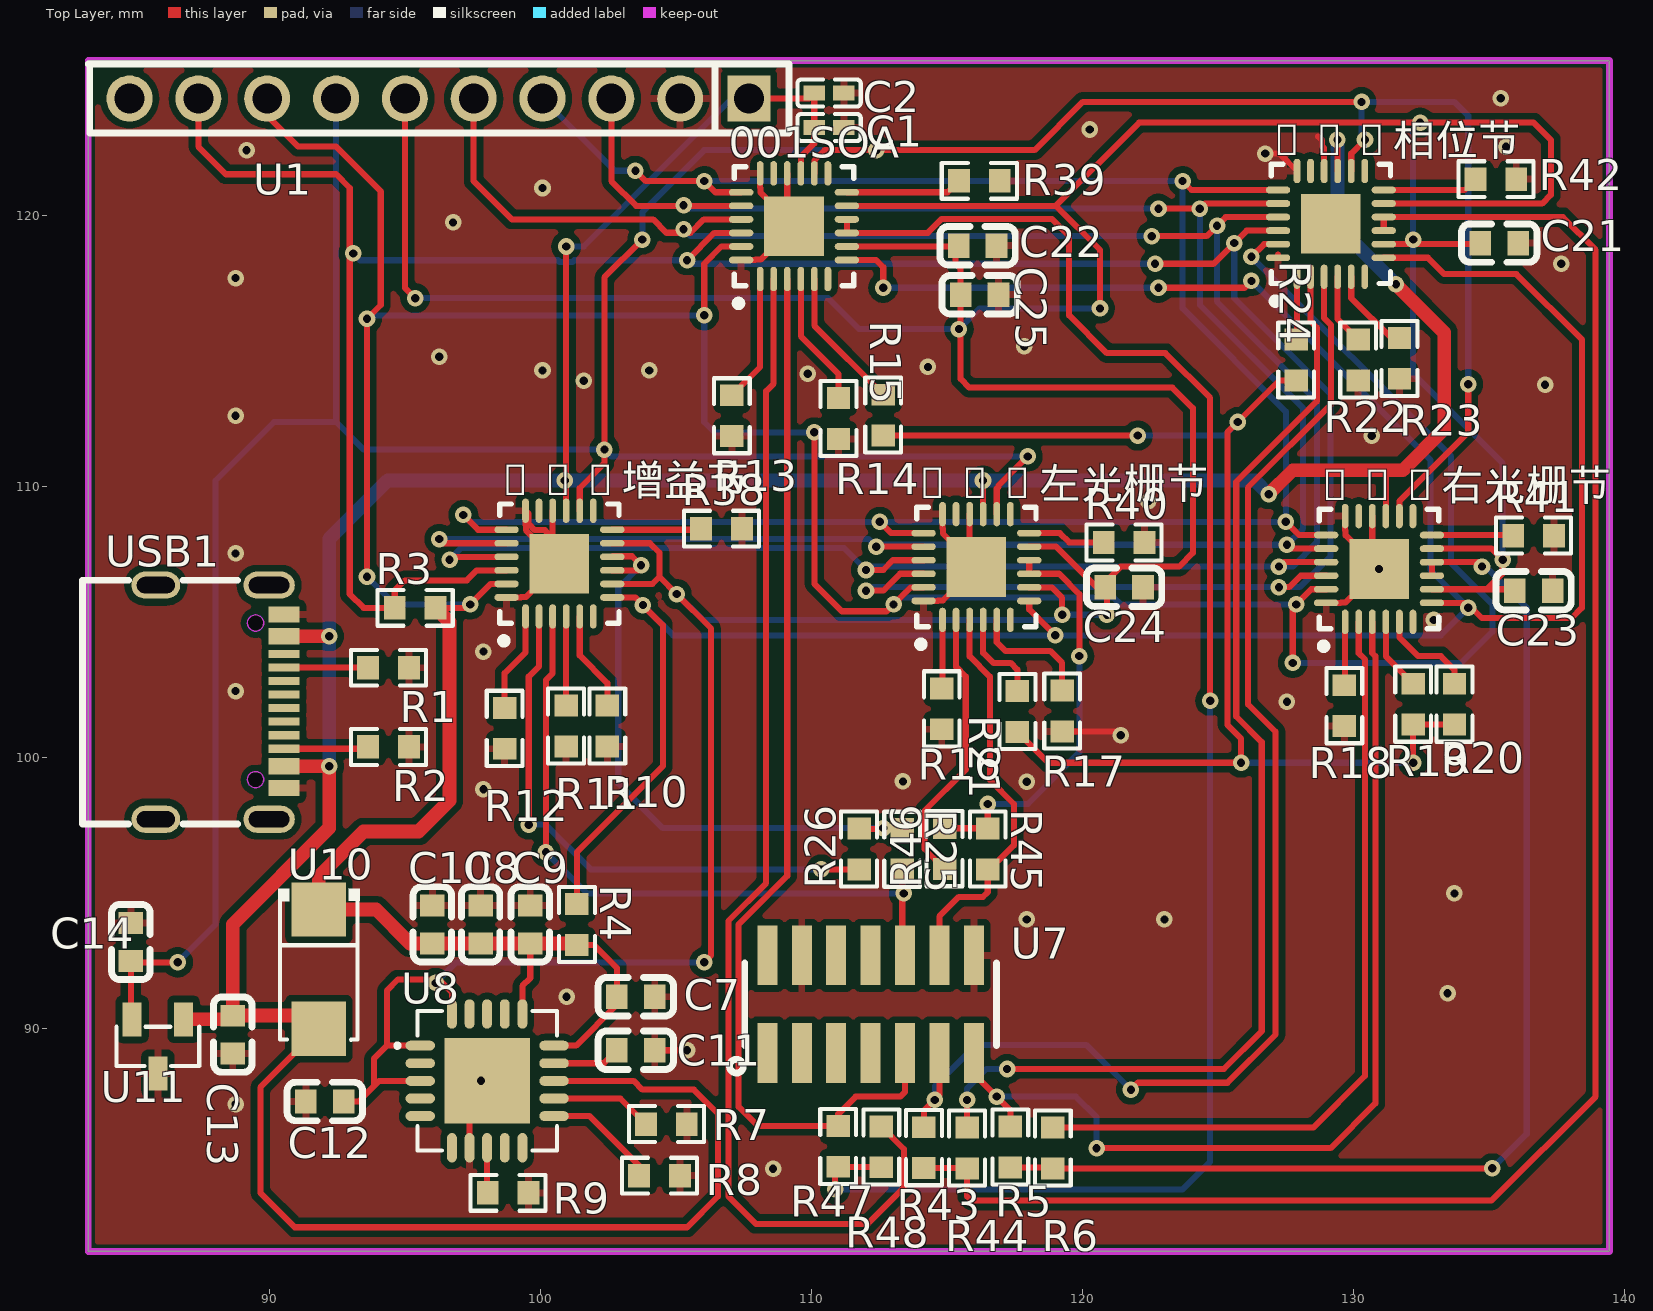
[diagram p0: Top Layer view]
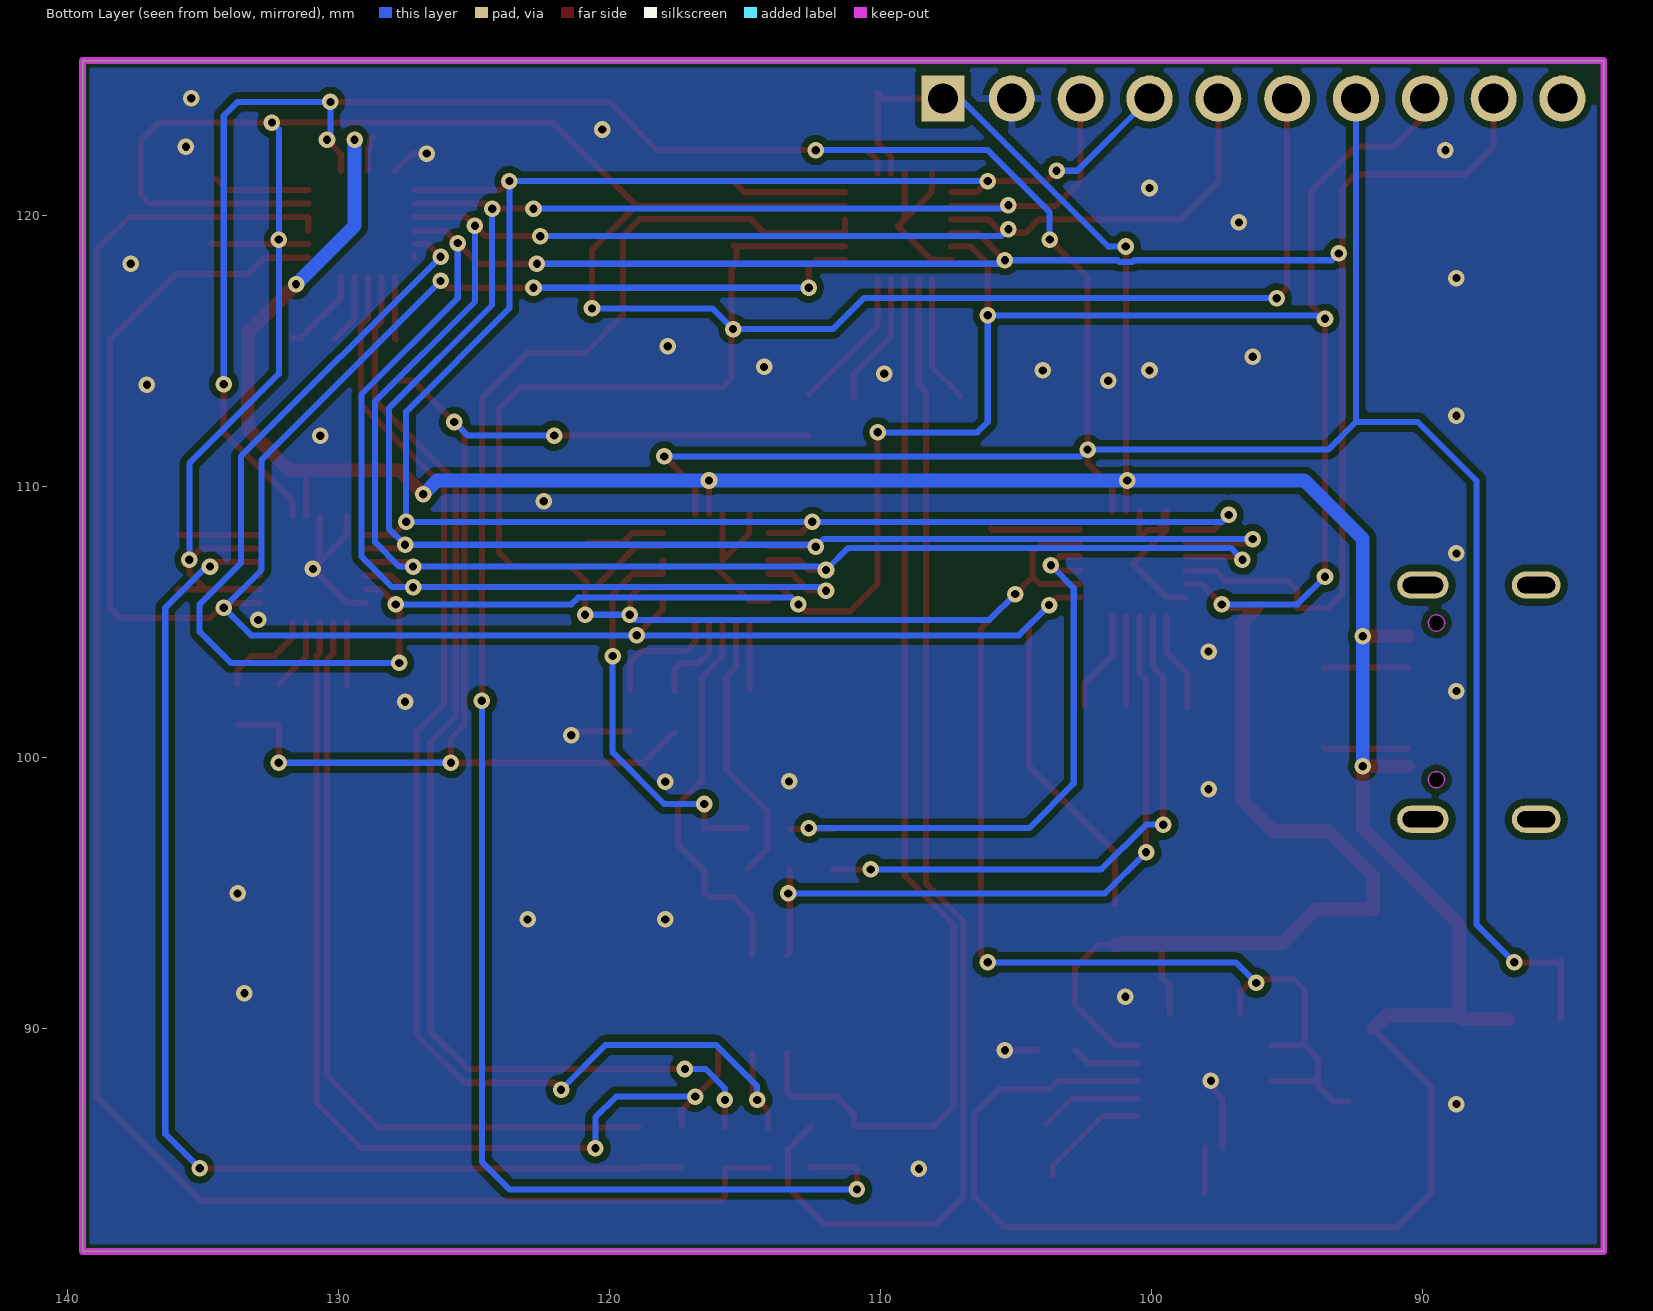
[diagram p1: Bottom Layer view, seen from below]
# Altium PCB MISC49910.pcbdoc
Units mm, origin at the board's own origin, x right, y up, seen from the top; angles counter-clockwise.
Board outline 56.13 x 43.94 mm, 2 copper layers (Top Layer, Bottom Layer), stack 1.58 mm thick; 63 components, 53 nets, 295 pads, 127 vias.

## Layer stack, top to bottom
Top Solder Mask Layer: solder mask 0.01, Dk 3.3
Top Layer: signal copper 0.035
Dielectric1: surface 1.51, FR4, Dk 4.5
Bottom Layer: signal copper 0.035
Bottom Solder Mask Layer: solder mask 0.01, Dk 3.3

## Board outline
83.312,125.73 83.312,81.788 139.446,81.788 139.446,125.73

## Design rules (kind name [scope] priority, off if disabled: settings)
BoardOutlineClearance copperThickness2oz_1 [All] p2 off: genericclearance=0.203 ignorepadtopadclearanceinfootprint=FALSE except(0: Arc-SplitContinuation Track-SplitContinuation SMDPad-SplitContinuation THPad-SplitContinuation Via-SplitContinuation Fill-SplitContinuation Region-SplitContinuation Poly-SplitContinuation Text-SplitContinuation Hole-SplitContinuation; 0.152: Arc-CutoutEdge SMDPad-CutoutEdge THPad-CutoutEdge Via-CutoutEdge Fill-CutoutEdge Region-CutoutEdge Text-CutoutEdge; 0.176: Hole-OutlineEdge Hole-CutoutEdge; 0.254: Poly-OutlineEdge Poly-CutoutEdge; 0.3: Arc-OutlineEdge Track-OutlineEdge SMDPad-OutlineEdge THPad-OutlineEdge Via-OutlineEdge Fill-OutlineEdge Region-OutlineEdge Text-OutlineEdge Track-CutoutEdge)
BoardOutlineClearance Plane_innerPlane_1 [All] p4 off: genericclearance=0.102 ignorepadtopadclearanceinfootprint=FALSE except(0: Arc-SplitContinuation Track-SplitContinuation SMDPad-SplitContinuation THPad-SplitContinuation Via-SplitContinuation Fill-SplitContinuation Region-SplitContinuation Poly-SplitContinuation Text-SplitContinuation Hole-SplitContinuation; 0.152: SMDPad-CutoutEdge THPad-CutoutEdge Via-CutoutEdge Fill-CutoutEdge Region-CutoutEdge Text-CutoutEdge; 0.176: Hole-OutlineEdge Hole-CutoutEdge; 0.254: Poly-OutlineEdge Poly-CutoutEdge; 0.3: Arc-OutlineEdge Track-OutlineEdge SMDPad-OutlineEdge THPad-OutlineEdge Via-OutlineEdge Fill-OutlineEdge Region-OutlineEdge Text-OutlineEdge Arc-CutoutEdge Track-CutoutEdge)
BoardOutlineClearance Copper_copperRegion_1 [All] p6 off: genericclearance=0.102 ignorepadtopadclearanceinfootprint=FALSE except(0: Arc-SplitContinuation Track-SplitContinuation SMDPad-SplitContinuation THPad-SplitContinuation Via-SplitContinuation Fill-SplitContinuation Region-SplitContinuation Poly-SplitContinuation Text-SplitContinuation Hole-SplitContinuation; 0.152: SMDPad-CutoutEdge THPad-CutoutEdge Via-CutoutEdge Fill-CutoutEdge Region-CutoutEdge Text-CutoutEdge; 0.176: Hole-OutlineEdge Hole-CutoutEdge; 0.254: Poly-OutlineEdge Poly-CutoutEdge; 0.3: Arc-OutlineEdge Track-OutlineEdge SMDPad-OutlineEdge THPad-OutlineEdge Via-OutlineEdge Fill-OutlineEdge Region-OutlineEdge Text-OutlineEdge Arc-CutoutEdge Track-CutoutEdge)
BoardOutlineClearance Copper_copperRegion_copperThickness1oz_1 [All] p8 off: genericclearance=0.102 ignorepadtopadclearanceinfootprint=FALSE except(0: Arc-SplitContinuation Track-SplitContinuation SMDPad-SplitContinuation THPad-SplitContinuation Via-SplitContinuation Fill-SplitContinuation Region-SplitContinuation Poly-SplitContinuation Text-SplitContinuation Hole-SplitContinuation; 0.152: SMDPad-CutoutEdge THPad-CutoutEdge Via-CutoutEdge Fill-CutoutEdge Region-CutoutEdge Text-CutoutEdge; 0.176: Hole-OutlineEdge Hole-CutoutEdge; 0.254: Poly-OutlineEdge Poly-CutoutEdge; 0.3: Arc-OutlineEdge Track-OutlineEdge SMDPad-OutlineEdge THPad-OutlineEdge Via-OutlineEdge Fill-OutlineEdge Region-OutlineEdge Text-OutlineEdge Arc-CutoutEdge Track-CutoutEdge)
BoardOutlineClearance Copper_copperRegion_Copper_copperRegion_1 [All] p10 off: genericclearance=0.102 ignorepadtopadclearanceinfootprint=FALSE except(0: Arc-SplitContinuation Track-SplitContinuation SMDPad-SplitContinuation THPad-SplitContinuation Via-SplitContinuation Fill-SplitContinuation Region-SplitContinuation Poly-SplitContinuation Text-SplitContinuation Hole-SplitContinuation; 0.152: SMDPad-CutoutEdge THPad-CutoutEdge Via-CutoutEdge Fill-CutoutEdge Region-CutoutEdge Text-CutoutEdge; 0.176: Hole-OutlineEdge Hole-CutoutEdge; 0.254: Poly-OutlineEdge Poly-CutoutEdge; 0.3: Arc-OutlineEdge Track-OutlineEdge SMDPad-OutlineEdge THPad-OutlineEdge Via-OutlineEdge Fill-OutlineEdge Region-OutlineEdge Text-OutlineEdge Arc-CutoutEdge Track-CutoutEdge)
BoardOutlineClearance copperThickness1oz_1 [All] p12: genericclearance=0.102 ignorepadtopadclearanceinfootprint=FALSE except(0: Arc-SplitContinuation Track-SplitContinuation SMDPad-SplitContinuation THPad-SplitContinuation Via-SplitContinuation Fill-SplitContinuation Region-SplitContinuation Poly-SplitContinuation Text-SplitContinuation Hole-SplitContinuation; 0.152: SMDPad-CutoutEdge THPad-CutoutEdge Via-CutoutEdge Fill-CutoutEdge Region-CutoutEdge Text-CutoutEdge; 0.176: Hole-OutlineEdge Hole-CutoutEdge; 0.254: Poly-OutlineEdge Poly-CutoutEdge; 0.3: Arc-OutlineEdge Track-OutlineEdge SMDPad-OutlineEdge THPad-OutlineEdge Via-OutlineEdge Fill-OutlineEdge Region-OutlineEdge Text-OutlineEdge Arc-CutoutEdge Track-CutoutEdge)
Clearance copperThickness2oz [All] p1 off: gap=0.203 ignorepadtopadclearanceinfootprint=FALSE except(0.152: SMDPad-Track SMDPad-SMDPad THPad-Track SMDPad-THPad THPad-THPad Track-Via SMDPad-Via THPad-Via Via-Via Fill-Track Region-Track Fill-SMDPad Region-SMDPad Fill-THPad Region-THPad Fill-Via Region-Via Fill-Fill Fill-Region Region-Region Arc-Track Arc-SMDPad Arc-THPad Arc-Via Fill-Arc Region-Arc Arc-Arc Text-Track SMDPad-Text Text-THPad Text-Via Fill-Text Region-Text Arc-Text Text-Text; 0.176: Hole-Track Hole-SMDPad Hole-THPad Hole-Via Fill-Hole Region-Hole Hole-Arc Hole-Text; 0.254: Poly-Track Poly-SMDPad Poly-THPad Poly-Via Poly-Fill Poly-Region Poly-Poly Poly-Arc Poly-Text Poly-Hole)
Clearance Plane_innerPlane [All] p3 off: gap=0.102 ignorepadtopadclearanceinfootprint=FALSE except(0.152: SMDPad-Track SMDPad-SMDPad THPad-Track SMDPad-THPad THPad-THPad Track-Via SMDPad-Via THPad-Via Via-Via Fill-Track Region-Track Fill-SMDPad Region-SMDPad Fill-THPad Region-THPad Fill-Via Region-Via Fill-Fill Fill-Region Region-Region Arc-Track Arc-SMDPad Arc-THPad Arc-Via Fill-Arc Region-Arc Arc-Arc Text-Track SMDPad-Text Text-THPad Text-Via Fill-Text Region-Text Arc-Text Text-Text; 0.176: Hole-Track Hole-SMDPad Hole-THPad Hole-Via Fill-Hole Region-Hole Hole-Arc Hole-Text; 0.254: Poly-Track Poly-SMDPad Poly-THPad Poly-Via Poly-Fill Poly-Region Poly-Poly Poly-Arc Poly-Text Poly-Hole)
Clearance Copper_copperRegion [All] p5 off: gap=0.102 ignorepadtopadclearanceinfootprint=FALSE except(0.152: SMDPad-Track SMDPad-SMDPad THPad-Track SMDPad-THPad THPad-THPad Track-Via SMDPad-Via THPad-Via Via-Via Fill-Track Region-Track Fill-SMDPad Region-SMDPad Fill-THPad Region-THPad Fill-Via Region-Via Fill-Fill Fill-Region Region-Region Arc-Track Arc-SMDPad Arc-THPad Arc-Via Fill-Arc Region-Arc Arc-Arc Text-Track SMDPad-Text Text-THPad Text-Via Fill-Text Region-Text Arc-Text Text-Text; 0.176: Hole-Track Hole-SMDPad Hole-THPad Hole-Via Fill-Hole Region-Hole Hole-Arc Hole-Text; 0.254: Poly-Track Poly-SMDPad Poly-THPad Poly-Via Poly-Fill Poly-Region Poly-Poly Poly-Arc Poly-Text Poly-Hole)
Clearance Copper_copperRegion_copperThickness1oz [All] p7 off: gap=0.102 ignorepadtopadclearanceinfootprint=FALSE except(0.152: SMDPad-Track SMDPad-SMDPad THPad-Track SMDPad-THPad THPad-THPad Track-Via SMDPad-Via THPad-Via Via-Via Fill-Track Region-Track Fill-SMDPad Region-SMDPad Fill-THPad Region-THPad Fill-Via Region-Via Fill-Fill Fill-Region Region-Region Arc-Track Arc-SMDPad Arc-THPad Arc-Via Fill-Arc Region-Arc Arc-Arc Text-Track SMDPad-Text Text-THPad Text-Via Fill-Text Region-Text Arc-Text Text-Text; 0.176: Hole-Track Hole-SMDPad Hole-THPad Hole-Via Fill-Hole Region-Hole Hole-Arc Hole-Text; 0.254: Poly-Track Poly-SMDPad Poly-THPad Poly-Via Poly-Fill Poly-Region Poly-Poly Poly-Arc Poly-Text Poly-Hole)
Clearance Copper_copperRegion_Copper_copperRegion [All] p9 off: gap=0.102 ignorepadtopadclearanceinfootprint=FALSE except(0.152: SMDPad-Track SMDPad-SMDPad THPad-Track SMDPad-THPad THPad-THPad Track-Via SMDPad-Via THPad-Via Via-Via Fill-Track Region-Track Fill-SMDPad Region-SMDPad Fill-THPad Region-THPad Fill-Via Region-Via Fill-Fill Fill-Region Region-Region Arc-Track Arc-SMDPad Arc-THPad Arc-Via Fill-Arc Region-Arc Arc-Arc Text-Track SMDPad-Text Text-THPad Text-Via Fill-Text Region-Text Arc-Text Text-Text; 0.176: Hole-Track Hole-SMDPad Hole-THPad Hole-Via Fill-Hole Region-Hole Hole-Arc Hole-Text; 0.254: Poly-Track Poly-SMDPad Poly-THPad Poly-Via Poly-Fill Poly-Region Poly-Poly Poly-Arc Poly-Text Poly-Hole)
Clearance copperThickness1oz [All] p11: gap=0.102 ignorepadtopadclearanceinfootprint=FALSE except(0.152: SMDPad-Track SMDPad-SMDPad THPad-Track SMDPad-THPad THPad-THPad Track-Via SMDPad-Via THPad-Via Via-Via Fill-Track Region-Track Fill-SMDPad Region-SMDPad Fill-THPad Region-THPad Fill-Via Region-Via Fill-Fill Fill-Region Region-Region Arc-Track Arc-SMDPad Arc-THPad Arc-Via Fill-Arc Region-Arc Arc-Arc Text-Track SMDPad-Text Text-THPad Text-Via Fill-Text Region-Text Arc-Text Text-Text; 0.176: Hole-Track Hole-SMDPad Hole-THPad Hole-Via Fill-Hole Region-Hole Hole-Arc Hole-Text; 0.254: Poly-Track Poly-SMDPad Poly-THPad Poly-Via Poly-Fill Poly-Region Poly-Poly Poly-Arc Poly-Text Poly-Hole)
DiffPairsRouting differentialPair [All] p1: maxlimit=0.152 minlimit=0.152 mostfreqgap=0.152 toplayer_minwidth=0.127 toplayer_prefwidth=0.254 toplayer_maxwidth=2.54 toplayer_mingap=0.152 toplayer_prefgap=0.152 toplayer_maxgap=0.152 bottomlayer_minwidth=0.127 bottomlayer_prefwidth=0.254 bottomlayer_maxwidth=2.54 bottomlayer_mingap=0.152 bottomlayer_prefgap=0.152 bottomlayer_maxgap=0.152 maxuncoupledlength=0.254
HoleToHoleClearance otherClearance [All] p1: gap=0.3 allowstackedmicrovias=TRUE
Length netLength [All] p1: minlimit=0 maxlimit=0
PasteMaskExpansion pasteMaskExpansion [All] p1: expansion=0
PlaneConnect innerPlane [All] p1: planeconnectstyle=Relief reliefexpansion=0.508 reliefentries=4 reliefconductorwidth=0.254 reliefairgap=0.254
PolygonConnect copperRegion_copperThickness1oz [All] p1 off: connectstyle=Relief reliefconductorwidth=0.254 reliefentries=4 polygonreliefangle="90 Angle" airgapwidth=0.254 via.connectstyle=Relief via.reliefconductorwidth=0.254 via.reliefentries=4 via.polygonreliefangle="90 Angle" via.airgapwidth=0.254
PolygonConnect copperRegion_Copper_copperRegion [All] p2 off: connectstyle=Relief reliefconductorwidth=0.254 reliefentries=4 polygonreliefangle="90 Angle" airgapwidth=0.254 via.connectstyle=Relief via.reliefconductorwidth=0.254 via.reliefentries=4 via.polygonreliefangle="90 Angle" via.airgapwidth=0.254
PolygonConnect copperRegion [All] p3: connectstyle=Relief reliefconductorwidth=0.254 reliefentries=4 polygonreliefangle="90 Angle" airgapwidth=0.254 via.connectstyle=Relief via.reliefconductorwidth=0.254 via.reliefentries=4 via.polygonreliefangle="90 Angle" via.airgapwidth=0.254
RoutingVias viaSize [All] p1: holewidth=0.305 width=0.61 viastyle="Through Hole" minholewidth=0.3 minwidth=0.5 maxholewidth=6.3 maxwidth=10
SolderMaskExpansion solderMaskExpansion [IsVia] p1: expansion=-25.4 istentingtop=TRUE
SolderMaskExpansion solderMaskExpansion [All] p2: expansion=0.051 istentingtop=FALSE
Width copperThickness2oz_2 [All] p1 off: maxlimit=2.54 minlimit=0.203 preferedwidth=0.254
Width copperThickness1oz_2 [All] p2: maxlimit=2.54 minlimit=0.127 preferedwidth=0.254

## Components (designator, comment, footprint, x,y, rotation, side; value= is the part's Value field where it differs from the comment)
000增益节 "ADN8810ACPZ" LFCSP-24_L4.0-W4.0-P0.50-BL-EP2.3 100.7,107.171 r0 top
001SOA "ADN8810ACPZ" LFCSP-24_L4.0-W4.0-P0.50-BL-EP2.3 109.358,119.623 r0 top
010左光栅节 "ADN8810ACPZ" LFCSP-24_L4.0-W4.0-P0.50-BL-EP2.3 116.089,107.044 r0 top
011右光栅节 "ADN8810ACPZ" LFCSP-24_L4.0-W4.0-P0.50-BL-EP2.3 130.948,106.973 r0 top
100相位节 "ADN8810ACPZ" LFCSP-24_L4.0-W4.0-P0.50-BL-EP2.3 129.17,119.708 r0 top
C1 "10uF" C0402 110.65,123.265 r180 top
C2 "100nF" C0402 110.65,124.535 r180 top
C7 "10uF" C0603 103.52,91.186 r0 top
C8 "10uF" C0603 97.79,93.853 r90 top
C9 "0.1uF" C0603 99.623,93.853 r270 top
C10 "0.1uF" C0603 96.012,93.853 r270 top
C11 "1uF" C0603 103.52,89.209 r180 top
C12 "10uF" C0603 92.043,87.319 r0 top
C13 "2.2uF" C0603 88.646,89.789 r270 top
C14 "2.2uF" C0603 84.884,93.206 r270 top
C21 "100nF" C0603 135.382,118.999 r0 top
C22 "100nF" C0603 116.132,118.903 r0 top
C23 "100nF" C0603 136.652,106.172 r0 top
C24 "100nF" C0603 121.539,106.299 r0 top
C25 "100nF" C0603 116.205,117.094 r0 top
R1 "5.1K" R0603 94.394,103.326 r180 top
R2 "5.1K" R0603 94.394,100.405 r180 top
R3 "10K" R0603 95.377,105.537 r0 top
R4 "10K" R0603 101.346,93.853 r270 top
R5 "3" R0603 117.34,85.637 r90 top
R6 "3" R0603 118.911,85.606 r270 top
R7 "0" R0603 104.648,86.487 r0 top
R8 "0" R0603 104.394,84.582 r0 top
R9 "0" R0603 98.806,83.947 r0 top
R10 "10K" R0603 102.469,101.176 r90 top
R11 "10K" R0603 100.945,101.176 r90 top
R12 "10K" R0603 98.679,101.092 r90 top
R13 "10K" R0603 107.063,112.627 r90 top
R14 "10K" R0603 110.998,112.522 r90 top
R15 "10K" R0603 112.649,112.649 r90 top
R16 "10K" R0603 114.81,101.811 r90 top
R17 "10K" R0603 119.253,101.727 r90 top
R18 "10K" R0603 129.669,101.925 r90 top
R19 "10K" R0603 132.207,101.981 r90 top
R20 "10K" R0603 133.731,101.981 r90 top
R21 "10K" R0603 117.602,101.71 r90 top
R22 "10K" R0603 130.175,114.681 r90 top
R23 "10K" R0603 131.701,114.744 r90 top
R24 "10K" R0603 127.889,114.681 r90 top
R25 "1.37" R0603 113.351,96.629 r270 top
R26 "1.37" R0603 111.758,96.64 r90 top
R38 "10K" R0603 106.68,108.458 r0 top
R39 "10K" R0603 116.196,121.294 r0 top
R40 "10K" R0603 121.539,107.95 r0 top
R41 "10K" R0603 136.652,108.204 r0 top
R42 "10K" R0603 135.26,121.358 r0 top
R43 "3" R0603 114.152,85.616 r90 top
R44 "3" R0603 115.744,85.605 r270 top
R45 "3" R0603 116.506,96.639 r270 top
R46 "3" R0603 114.914,96.65 r90 top
R47 "1.37" R0603 110.986,85.663 r90 top
R48 "1.37" R0603 112.579,85.646 r270 top
U1 "2.54mm pitch red header 1x10pin" HDR-TH_10P-P2.54-V-F-2 96.266,124.333 r180 top
U7 "ATLS7503" HDR-SMD_14P-P1.27-V-F-R2-C7-LS4.8 112.185,90.91 r0 top
U8 "TPS7A4701RGWR" VQFN-20_L5.0-W5.0-P0.65-TL-EP 98.033,88.081 r0 top
U10 "SS310 Schottky diode SMA" SMA_L4.3-W2.6-LS5.1-R-RD 91.821,92.202 r270 top
U11 "REF2940AIDBZT" SOT-23-3_L2.9-W1.3-P1.90-LS2.4-BR 85.881,89.352 r90 top
USB1 "Type-C-16P" USB-C-SMD_GT-USB-7010E 88.171,102.056 r270 top

## Footprints (in the part's own frame and the unit in brackets; to place one, negate y for a bottom-side part, rotate by r counter-clockwise, add the part's x,y. Pads: shape width x height; smd on the part's side, far side on the other; paste and mask are expansions set on the pad)
C0402 [mm]
  rect 0.79x0.54 smd paste-100 mask+0.051: 1(-0.545,0) 2(0.545,0)
  silkscreen extent -1.17,-0.5 1.17,0.5
C0603 [mm]
  rect 0.8x0.9 smd: 1(-0.7,0) 2(0.7,0)
  silkscreen extent -1.39,-0.71 1.39,0.71
HDR-SMD_14P-P1.27-V-F-R2-C7-LS4.8 [mm]
  rect 0.74x2.2 smd: 1(-3.81,-1.8) 2(-3.81,1.8) 3(-2.54,-1.8) 4(-2.54,1.8) 5(-1.27,-1.8) 6(-1.27,1.8) 7(0,-1.8) 8(0,1.8) 9(1.27,-1.8) 10(1.27,1.8) 11(2.54,-1.8) 12(2.54,1.8) 13(3.81,-1.8) 14(3.81,1.8)
  silkscreen extent -5.21,-2.54 4.64,1.52
HDR-TH_10P-P2.54-V-F-2 [mm]
  rect 1.575x1.7 hole 1.1: 1(-11.43,0)
  round 1.7 hole 1.1: 2(-8.89,0) 3(-6.35,0) 4(-3.81,0) 5(-1.27,0) 6(1.27,0) 7(3.81,0) 8(6.35,0) 9(8.89,0) 10(11.43,0)
  silkscreen extent -12.9,-1.27 12.95,1.27
LFCSP-24_L4.0-W4.0-P0.50-BL-EP2.3 [mm]
  oval 0.25x0.9 smd paste-100 mask+0.05: 1(-1.25,-1.951) 2(-0.75,-1.951) 3(-0.25,-1.951) 4(0.25,-1.951) 5(0.75,-1.951) 6(1.25,-1.951) 13(1.25,1.951) 14(0.75,1.951) 15(0.25,1.951) 16(-0.25,1.951) 17(-0.75,1.951) 18(-1.25,1.951)
  oval 0.9x0.25 smd paste-100 mask+0.05: 7(1.951,-1.25) 8(1.951,-0.75) 9(1.951,-0.25) 10(1.951,0.25) 11(1.951,0.75) 12(1.951,1.25) 19(-1.951,1.25) 20(-1.951,0.75) 21(-1.951,0.25) 22(-1.951,-0.25) 23(-1.951,-0.75) 24(-1.951,-1.25)
  rect 2.2x2.2 smd paste-100 mask+0.05: 25(0,0)
  silkscreen extent -2.2,-2.98 2.2,2.2
R0603 [mm]
  rect 0.806x0.864 smd paste-100 mask+0.051: 1(-0.753,0) 2(0.753,0)
  silkscreen extent -1.39,-0.66 1.39,0.66
SMA_L4.3-W2.6-LS5.1-R-RD [mm]
  rect 2x2 smd: 1(2.2,0) 2(-2.2,0)
  silkscreen extent -2.98,-1.5 2.6,1.5
SOT-23-3_L2.9-W1.3-P1.90-LS2.4-BR [mm]
  rect 1.25x0.7 smd: 1(1,-0.95) 2(1,0.95) 3(-1,0)
  silkscreen extent -0.73,-1.53 0.73,1.53
USB-C-SMD_GT-USB-7010E [mm]
  oval 1x1.9 hole 0.6 slot 1.5 at 90 deg paste+0 mask+0.05: 1(-4.32,1.815) 2(4.32,1.815)
  oval 1x1.8 hole 0.6 slot 1.4 at 90 deg paste+0 mask+0.05: 3(4.32,-2.365) 4(-4.32,-2.365)
  rect 0.6x1.15 smd paste-100 mask+0.05: A1B12(-3.232,2.365) A4B9(-2.432,2.365) B1A12(3.168,2.365) B4A9(2.368,2.365)
  rect 0.3x1.15 smd paste-100 mask+0.05: A5(-1.282,2.365) A6(-0.282,2.365) A7(0.218,2.365) A8(1.218,2.365) B5(1.718,2.365) B6(0.718,2.365) B7(-0.782,2.365) B8(-1.782,2.365)
  Board Outline Layer circle w0.003: c2.858,1.315 r0.3
  Board Outline Layer circle w0.003: c-2.922,1.315 r0.3
  Board Outline Layer region: 2.858,1.615 2.988,1.585 3.093,1.502 3.15,1.382 3.15,1.248 3.093,1.128 2.988,1.045 2.858,1.015 2.858,1.015 2.728,1.045 2.623,1.128 2.566,1.248 2.566,1.382 2.623,1.502 2.728,1.585 2.858,1.615
  Board Outline Layer region: 2.858,1.615 2.93,1.606 2.997,1.581 3.057,1.54 3.105,1.485 3.139,1.421 3.156,1.351 3.156,1.279 3.139,1.209 3.105,1.145 3.057,1.09 2.997,1.049 2.93,1.024 2.858,1.015 2.786,1.024 2.719,1.049 2.659,1.09 2.611,1.145 2.578,1.209 2.56,1.279 2.56,1.351 2.578,1.421 2.611,1.485 2.659,1.54 2.719,1.581 2.786,1.606
  Board Outline Layer region: -2.922,1.615 -2.792,1.585 -2.687,1.502 -2.63,1.382 -2.63,1.248 -2.687,1.128 -2.792,1.045 -2.922,1.015 -2.922,1.015 -3.052,1.045 -3.157,1.128 -3.214,1.248 -3.214,1.382 -3.157,1.502 -3.052,1.585 -2.922,1.615
  Board Outline Layer region: -2.922,1.615 -2.85,1.606 -2.783,1.581 -2.723,1.54 -2.675,1.485 -2.642,1.421 -2.624,1.351 -2.624,1.279 -2.642,1.209 -2.675,1.145 -2.723,1.09 -2.783,1.049 -2.85,1.024 -2.922,1.015 -2.994,1.024 -3.061,1.049 -3.121,1.09 -3.169,1.145 -3.203,1.209 -3.22,1.279 -3.22,1.351 -3.203,1.421 -3.169,1.485 -3.121,1.54 -3.061,1.581 -2.994,1.606
  Multi-Layer board cut-out: 2.858,1.615 2.988,1.585 3.093,1.502 3.15,1.382 3.15,1.248 3.093,1.128 2.988,1.045 2.858,1.015 2.858,1.015 2.728,1.045 2.623,1.128 2.566,1.248 2.566,1.382 2.623,1.502 2.728,1.585 2.858,1.615
  Multi-Layer board cut-out: -2.922,1.615 -2.792,1.585 -2.687,1.502 -2.63,1.382 -2.63,1.248 -2.687,1.128 -2.792,1.045 -2.922,1.015 -2.922,1.015 -3.052,1.045 -3.157,1.128 -3.214,1.248 -3.214,1.382 -3.157,1.502 -3.052,1.585 -2.922,1.615
  silkscreen extent -4.5,-5.07 4.5,0.66
VQFN-20_L5.0-W5.0-P0.65-TL-EP [mm]
  oval 1.087x0.364 smd paste-100 mask+0.051: 1(-2.468,1.3) 2(-2.468,0.65) 3(-2.468,0) 4(-2.468,-0.65) 5(-2.468,-1.3) 11(2.468,-1.3) 12(2.468,-0.65) 13(2.468,0) 14(2.468,0.65) 15(2.468,1.3)
  oval 0.364x1.087 smd paste-100 mask+0.051: 6(-1.3,-2.468) 7(-0.65,-2.468) 8(0,-2.468) 9(0.65,-2.468) 10(1.3,-2.468) 16(1.3,2.468) 17(0.65,2.468) 18(0,2.468) 19(-0.65,2.468) 20(-1.3,2.468)
  rect 3.15x3.15 smd paste-100 mask+0.051: 21(0,0)
  silkscreen extent -3.39,-2.58 2.58,2.58

## Via types
v1: diameter 0.61, hole 0.305, Top Layer to Bottom Layer, 127 vias

## Nets (pads, with @x,y where several pads share a name; then routed paths per layer and width w, separated by ;. In a path a pad name is that pad's centre, name@x,y a point inside that pad or via, vN(x,y) a via of type N, cw(c..) or ccw(c..) an arc to the next point about the centre after c; other vN are vias at no path point)
3.3V_ANA: 000增益节.8 000增益节.11 001SOA.8 001SOA.11 010左光栅节.8 010左光栅节.11 011右光栅节.8 011右光栅节.11 100相位节.8 100相位节.11 C12.2 C21.1 C22.1 C23.1 C24.1 C25.1 U1.6 U8.1 U8.3 U8.20 | length 194.1
  Top Layer w0.225: C12.2 93.288,87.319 93.853,87.884 ; U1.6 94.996,117.348 v1(95.377,116.967) ; U8.3 94.05,88.081 93.853,87.884 ; U8.1 94.334,89.381 ; U8.20 96.733,91.354 96.266,91.821 94.742,91.821 94.334,91.413 94.334,89.381 ; 000增益节.8 104.135,106.421 104.394,106.68 ; 000增益节.11 104.042,107.921 104.394,107.569 104.394,106.68 ; v1(106.045,92.456) 106.299,92.71 106.299,104.775 v1(105.029,106.045) 104.394,106.68 ; 001SOA.8 C22.1@115.402,118.872 ; 001SOA.11 119.022,120.373 ; C22.1 C22.1@115.402,118.872 ; 010左光栅节.8 118.877,106.294 119.253,105.918 v1(119.253,105.283) ; 010左光栅节.11 119.028,107.794 120.528,106.294 120.834,106.294 C24.1 ; v1(120.65,116.586) 120.65,118.745 119.022,120.373 ; v1(120.904,105.283) 120.904,106.234 C24.1 ; 100相位节.8 134.64,118.957 C21.1 ; 100相位节.11 136.968,120.458 137.287,120.777 137.287,122.809 136.652,123.444 v1(132.461,123.444) 122.093,123.444 119.022,120.373 ; 011右光栅节.8 134.925,106.222 ; 011右光栅节.11 135.101,107.723 v1(135.509,107.315) 135.509,106.807 134.925,106.222 ; C23.1 135.902,106.222 134.925,106.222 ; 93.853,87.884 93.853,88.9 94.334,89.381 ; C22.1@115.402,118.872 115.316,118.787 115.316,118.237 115.505,118.048 C25.1 115.505,113.984 115.824,113.665 123.317,113.665 124.079,112.903 124.079,107.569 123.571,107.061 121.412,107.061 120.839,106.488 C24.1
  Bottom Layer w0.225: v1(95.377,116.967) 110.617,116.967 111.76,115.824 v1(115.443,115.824) 116.205,116.586 v1(120.65,116.586) ; v1(96.139,91.694) 96.901,92.456 v1(106.045,92.456) ; v1(105.029,106.045) 105.983,105.091 119.061,105.091 v1(119.253,105.283) v1(120.904,105.283) ; v1(132.461,123.444) 132.207,123.19 v1(132.207,119.126) 132.207,114.173 135.509,110.871 v1(135.509,107.315)
3V3_OUT: R15.1 R19.1 R20.1 R21.1 R24.1 | length 47
  Top Layer w0.225: R15.1 v1(122.047,111.896) ; R21.1 118.736,99.822 v1(125.857,99.822) 125.857,100.711 125.349,101.219 125.349,112.014 v1(125.73,112.395) 127.263,113.928 R24.1 ; v1(132.207,99.822) R19.1 R20.1
  Bottom Layer w0.225: v1(122.047,111.896) 125.231,111.896 v1(125.73,112.395) ; v1(125.857,99.822) v1(132.207,99.822)
$1N135: 000增益节.12 R38.1 | length 3.3
  Top Layer w0.225: 000增益节.12 105.889,108.421 R38.1
$1N144: 000增益节.5 R10.2 | length 3.7
  Top Layer w0.225: 000增益节.5 101.45,103.782 102.469,102.763 R10.2
$1N160: 001SOA.5 R15.2 | length 5.3
  Top Layer w0.225: 001SOA.5 110.108,115.952 112.649,113.411 R15.2
$1N162: 001SOA.12 R39.1 | length 4.3
  Top Layer w0.225: 001SOA.12 115.022,120.872 R39.1
$1N165: 010左光栅节.12 R40.1 | length 2.9
  Top Layer w0.225: 010左光栅节.12 119.163,108.294 119.507,107.95 R40.1
$1N177: 010左光栅节.5 R17.2 | length 4.6
  Top Layer w0.225: 010左光栅节.5 116.839,104.268 117.156,103.951 118.807,103.951 119.253,103.505 R17.2
$1N190: 011右光栅节.12 R41.1 | length 3
  Top Layer w0.225: 011右光栅节.12 135.88,108.222 R41.1
$1N192: 011右光栅节.5 R20.2 | length 3.6
  Top Layer w0.225: 011右光栅节.5 131.698,104.449 132.388,103.759 133.223,103.759 133.731,103.251 R20.2
$1N195: 100相位节.12 R42.1 | length 3.6
  Top Layer w0.225: 100相位节.12 134.106,120.957 R42.1
$1N203: 100相位节.5 R23.2 | length 3.2
  Top Layer w0.225: 100相位节.5 129.92,116.968 131.391,115.497 R23.2
$1N217: R9.1 U8.8 | length 1.7
  Top Layer w0.225: U8.8 98.033,83.967 R9.1
$1N219: R7.1 U8.12 | length 3.8
  Top Layer w0.225: U8.12 102.951,87.431 R7.1
$1N220: R8.1 U8.11 | length 4.3
  Top Layer w0.225: U8.11 101.814,86.781 103.641,84.954 R8.1
$1N222: C11.2 U8.14 | length 2.5
  Top Layer w0.225: U8.14 102.341,88.731 C11.2
$1N225: 000增益节.1 R12.2 | length 3.7
  Top Layer w0.225: R12.2 98.679,103.124 99.45,103.895 000增益节.1
$1N226: 000增益节.4 R11.2 | length 3.3
  Top Layer w0.225: R11.2 100.95,101.934 000增益节.4
$1N227: 001SOA.1 R13.2 | length 4.7
  Top Layer w0.225: R13.2 108.108,114.426 001SOA.1
$1N228: 001SOA.4 R14.2 | length 5
  Top Layer w0.225: 001SOA.4 109.608,115.563 110.998,114.173 R14.2
$1N231: 010左光栅节.1 R16.2 | length 2.5
  Top Layer w0.225: R16.2 114.839,102.594 010左光栅节.1
$1N233: 010左光栅节.4 R21.2 | length 3.5
  Top Layer w0.225: 010左光栅节.4 116.339,103.879 116.713,103.505 117.348,103.505 117.602,103.251 R21.2
$1N234: 011右光栅节.1 R18.2 | length 2.4
  Top Layer w0.225: R18.2 129.698,102.708 011右光栅节.1
$1N236: 011右光栅节.4 R19.2 | length 2.7
  Top Layer w0.225: 011右光栅节.4 131.198,103.752 132.207,102.743 R19.2
$1N240: 100相位节.4 R22.2 | length 2.6
  Top Layer w0.225: 100相位节.4 129.42,116.189 R22.2
$1N242: 100相位节.1 R24.2 | length 2.3
  Top Layer w0.225: R24.2 127.92,115.466 100相位节.1
$1N278: U7.5
$1N324: R1.2 USB1.A5 | length 3.1
  Top Layer w0.225: USB1.A5 93.629,103.338 R1.2
$1N326: R2.2 USB1.B5 | length 3.1
  Top Layer w0.225: USB1.B5 93.574,100.338 R2.2
+5V_IN: 000增益节.15 001SOA.15 010左光栅节.15 011右光栅节.15 100相位节.15 C1.2 C2.2 C13.1 U1.1 U8.13 U10.1 U11.1 USB1.A4B9 USB1.B4A9 | length 146.1
  Top Layer w0.225: U10.1 89.662,87.843 89.662,83.947 90.932,82.677 105.41,82.677 106.553,83.82 106.553,86.868 105.664,87.757 103.759,87.757 103.435,88.081 U8.13 ; 000增益节.15 v1(100.95,118.872) ; U1.1 109.904,124.333 C2.2 C1.2 110.105,122.678 109.608,122.181 001SOA.15 ; v1(116.332,110.236) 116.339,110.229 010左光栅节.15 ; v1(129.413,122.809) 129.42,122.802 100相位节.15 ; 131.191,110.617 131.198,110.61 011右光栅节.15
  Top Layer w0.508: U11.1 88.509,90.352 C13.1 ; USB1.B4A9 90.543,99.695 v1(92.202,99.695) 92.202,97.409 88.646,93.853 C13.1 ; USB1.A4B9 v1(92.202,104.488) ; U10.1 91.334,90.489 C13.1 ; v1(126.873,109.728) 127.762,110.617 131.191,110.617 131.826,110.617 133.35,112.141 133.35,115.697 v1(131.572,117.475)
  Bottom Layer w0.225: v1(100.95,118.872) 101.6,118.872 107.061,124.333 U1.1
  Bottom Layer w0.508: v1(92.202,99.695) v1(92.202,104.488) 92.202,108.077 94.361,110.236 v1(100.897,110.236) v1(116.332,110.236) 126.365,110.236 v1(126.873,109.728) ; v1(129.413,122.809) 129.413,119.634 v1(131.572,117.475)
ADN_CS_LASER: 000增益节.21 001SOA.21 010左光栅节.21 011右光栅节.21 100相位节.21 U1.5 | length 88.6
  Top Layer w0.225: v1(96.647,107.315) 96.753,107.421 000增益节.21 ; U1.5 97.536,121.285 98.948,119.873 104.155,119.873 104.648,119.38 105.537,119.38 106.03,119.873 001SOA.21 ; v1(112.014,106.934) 112.649,106.934 113.009,107.294 010左光栅节.21 ; v1(122.555,119.253) 124.587,119.253 v1(124.968,119.634) 125.292,119.958 100相位节.21 ; v1(127.254,107.061) 127.416,107.223 011右光栅节.21
  Bottom Layer w0.225: v1(96.647,107.315) 97.082,107.75 111.198,107.75 v1(112.014,106.934) 112.141,107.061 v1(127.254,107.061) 127.762,107.061 128.651,107.95 128.651,113.157 124.968,116.84 v1(124.968,119.634) ; v1(105.283,119.507) 105.537,119.253 v1(122.555,119.253)
ADN_SPI1_MOSI: 000增益节.19 001SOA.19 010左光栅节.19 011右光栅节.19 100相位节.19 U1.4 | length 80
  Top Layer w0.225: v1(97.155,108.966) 97.7,108.421 000增益节.19 ; v1(103.505,121.666) 103.886,121.285 v1(106.045,121.285) 106.458,120.872 001SOA.19 ; v1(112.522,108.712) 112.94,108.294 010左光栅节.19 ; v1(123.698,121.285) 124.026,120.957 100相位节.19 ; v1(127.508,108.712) 127.998,108.222 011右光栅节.19
  Bottom Layer w0.225: v1(97.155,108.966) 97.409,108.712 v1(112.522,108.712) v1(127.508,108.712) 127.508,112.776 123.698,116.586 v1(123.698,121.285) v1(106.045,121.285) ; U1.4 102.743,121.666 v1(103.505,121.666)
ADN_SPI1_SCK: 000增益节.20 001SOA.20 010左光栅节.20 011右光栅节.20 100相位节.20 U1.3 | length 81.7
  Top Layer w0.225: v1(96.266,108.077) 96.422,107.921 000增益节.20 ; U1.3 102.616,121.285 103.528,120.373 001SOA.20 ; v1(112.395,107.794) 010左光栅节.20 ; v1(122.809,120.269) v1(124.333,120.269) 124.522,120.458 100相位节.20 ; v1(127.55,107.865) 127.692,107.723 011右光栅节.20
  Bottom Layer w0.225: v1(96.266,108.077) 112.112,108.077 v1(112.395,107.794) 112.466,107.865 v1(127.55,107.865) 128.143,108.458 128.143,112.903 124.333,116.713 v1(124.333,120.269) ; v1(105.283,120.396) 105.41,120.269 v1(122.809,120.269)
DVDD: 000增益节.23 001SOA.23 010左光栅节.23 011右光栅节.23 100相位节.23 C7.1 C8.1 C9.2 C10.2 R3.2 R4.2 U1.8 U8.15 U8.16 U10.2 | length 140.8
  Top Layer w0.225: U1.8 89.916,123.698 91.059,122.555 92.456,122.555 94.107,120.904 94.107,116.713 v1(93.599,116.205) v1(93.599,106.68) ; R3.2 97.282,105.537 98.166,106.421 000增益节.23 ; U8.16 99.333,91.586 99.623,91.876 C9.2 ; U8.15 101.319,89.381 102.82,90.882 C7.1 102.82,92.252 101.972,93.1 R4.2 ; v1(106.045,116.332) 106.045,118.237 106.68,118.872 001SOA.23 ; v1(110.109,112.014) 110.109,106.426 111.125,105.41 112.776,105.41 v1(113.03,105.664) 113.66,106.294 010左光栅节.23 ; v1(126.238,118.491) 126.704,118.957 100相位节.23 ; v1(127.762,103.505) 127.762,105.537 v1(127.889,105.664) 128.447,106.222 011右光栅节.23
  Top Layer w0.508: R3.2 96.647,105.02 96.647,98.425 95.504,97.282 93.472,97.282 91.821,95.631 U10.2 93.939,94.402 95.188,93.153 C10.2 C8.1 C9.2 101.293,93.153 R4.2
  Bottom Layer w0.225: v1(93.599,106.68) 94.615,105.664 v1(97.409,105.664) ; v1(93.599,116.205) 93.726,116.332 v1(106.045,116.332) 106.045,112.395 106.426,112.014 v1(110.109,112.014) ; v1(113.03,105.664) 113.284,105.918 121.158,105.918 121.412,105.664 v1(127.889,105.664) ; v1(126.238,118.491) 133.604,111.125 133.604,107.188 135.128,105.664 135.128,104.648 133.985,103.505 v1(127.762,103.505)
FB1: 000增益节.3 R25.2 U7.10 | length 25.9
  Top Layer w0.225: v1(100.203,96.52) 100.203,102.87 100.45,103.117 000增益节.3 ; R25.2 113.351,92.815 U7.10
  Bottom Layer w0.225: v1(100.203,96.52) 101.727,94.996 v1(113.411,94.996)
FB2: 001SOA.3 R47.2 U7.9 | length 39.9
  Top Layer w0.225: 001SOA.3 109.108,95.646 107.315,93.853 107.315,87.122 108.021,86.416 R47.2 110.986,86.856 111.633,87.503 113.284,87.503 113.455,87.674 U7.9
FB3: 010左光栅节.3 R45.2 U7.12 | length 14.8
  Top Layer w0.225: U7.12 114.725,94.151 115.443,94.869 116.332,94.869 116.506,95.043 R45.2 116.587,95.886 117.475,96.774 117.475,98.298 116.586,99.187 116.586,102.997 115.839,103.744 010左光栅节.3
FB4: 011右光栅节.3 R5.2 U7.13 | length 37.2
  Top Layer w0.225: U7.13 115.995,88.348 v1(116.84,87.503) 117.34,87.003 R5.2 ; v1(120.523,85.598) 129.159,85.598 130.81,87.249 130.81,103.759 130.698,103.871 011右光栅节.3
  Bottom Layer w0.225: v1(116.84,87.503) 119.761,87.503 120.523,86.741 v1(120.523,85.598)
FB5: 100相位节.3 R43.2 U7.11 | length 48
  Top Layer w0.225: R43.2 114.152,86.974 114.725,87.547 U7.11 ; v1(121.793,87.757) 122.047,88.011 125.349,88.011 127.127,89.789 127.127,100.965 126.111,101.981 126.111,109.982 129.177,113.048 129.177,115.969 128.92,116.227 100相位节.3
  Bottom Layer w0.225: v1(114.554,87.376) 114.554,87.884 116.078,89.408 120.142,89.408 v1(121.793,87.757)
GND: 000增益节.16 000增益节.18 000增益节.24 000增益节.25 001SOA.16 001SOA.18 001SOA.24 001SOA.25 010左光栅节.16 010左光栅节.18 010左光栅节.24 010左光栅节.25 011右光栅节.16 011右光栅节.18 011右光栅节.24 011右光栅节.25 100相位节.16 100相位节.18 100相位节.24 C1.1 C2.1 C7.2 C8.2 C9.1 C10.1 C11.1 C12.1 C13.2 C14.1 C21.2 C22.2 C23.2 C24.2 C25.2 R1.1 R2.1 R7.2 R8.2 R9.2 R10.1 R11.1 R12.1 R13.1 R14.1 R16.1 R17.1 R18.1 R22.1 R23.1 R38.2 R39.2 R40.2 R41.2 R42.2 U1.2 U7.4 U7.14 U8.7 U8.21 U11.3 USB1.A1B12 USB1.B1A12 | length 36.2
  Top Layer w0.225: U8.7 97.383,87.431 U8.21 ; 000增益节.24 99.276,105.921 99.289,105.935 99.464,105.935 000增益节.25 99.464,108.407 99.464,108.582 99.45,108.595 000增益节.18 99.56,109.012 99.56,108.635 99.788,108.407 100.165,108.407 100.45,108.122 000增益节.16 ; C11.1 v1(105.41,89.209) ; 001SOA.24 107.934,118.373 107.947,118.386 108.122,118.386 001SOA.25 001SOA.25@109.108,119.873 ; 001SOA.18 108.108,121.047 108.122,121.034 108.122,120.859 001SOA.25@109.108,119.873 ; 001SOA.16 001SOA.25@109.108,119.873 ; 010左光栅节.24 114.665,105.794 114.678,105.808 114.853,105.808 010左光栅节.25 ; 010左光栅节.18 114.839,108.468 114.853,108.455 114.853,108.28 115.839,107.294 010左光栅节.16 ; R17.1 121.276,100.974 v1(121.412,100.838) ; v1(126.746,122.301) 127.278,122.301 100相位节.18 ; 100相位节.24 100相位节.24@127.219,118.568 ; 128.695,122.936 128.843,122.788 128.843,122.573 128.92,122.496 100相位节.16 ; 011右光栅节.24 129.524,105.723 129.537,105.736 129.712,105.736 v1(130.948,106.973) 011右光栅节.25@130.698,107.223 ; 011右光栅节.18 129.698,108.397 129.712,108.384 129.712,108.209 011右光栅节.25@130.698,107.223 ; 011右光栅节.16 011右光栅节.25@130.698,107.223
  other v1: 108.585,84.836 88.75,87.226 97.808,88.081 100.965,91.186 133.477,91.313 117.946,94.037 123.026,94.037 133.731,94.996 97.896,98.845 117.946,99.117 113.376,99.131 127.548,102.07 88.75,102.466 97.896,103.925 132.969,105.091 88.75,107.546 122.428,109.474 130.683,111.887 88.75,112.626 137.073,113.773 101.6,113.919 109.862,114.173 100.076,114.3 104.013,114.3 114.3,114.427 96.266,114.808 117.856,115.189 88.75,117.706 137.668,118.237 96.774,119.761 100.076,121.031 89.154,122.428 135.636,122.555 120.269,123.19 135.442,124.341
IOUT1: 000增益节.9 000增益节.10 R25.1 R26.2 | length 22.9
  Top Layer w0.225: 000增益节.9 103.619,106.921 103.712,107.014 v1(103.712,107.108) 103.378,107.442 102.672,107.442 000增益节.10 ; R26.2 111.769,97.383 R25.1
  Bottom Layer w0.225: v1(103.712,107.108) 102.87,106.267 102.87,99.06 104.521,97.409 v1(112.649,97.409)
IOUT2: 001SOA.9 001SOA.10 R47.1 R48.2 | length 63.5
  Top Layer w0.225: v1(110.871,84.074) 110.871,84.794 R47.1 112.562,84.91 R48.2 ; 001SOA.10 001SOA.9 114.293,119.373 114.808,119.888 118.872,119.888 119.507,119.253 119.507,116.332 120.904,114.935 123.063,114.935 124.714,113.284 v1(124.714,102.108)
  Bottom Layer w0.225: v1(110.871,84.074) 123.698,84.074 124.714,85.09 v1(124.714,102.108)
IOUT3: 010左光栅节.9 010左光栅节.10 R45.1 R46.2 | length 15.2
  Top Layer w0.225: R46.2 116.496,97.404 R45.1 v1(116.506,98.298) ; 010左光栅节.10 010左光栅节.9 119.139,106.794 119.888,106.045 v1(119.888,103.759)
  Bottom Layer w0.225: v1(116.506,98.298) 117.983,98.298 119.888,100.203 v1(119.888,103.759)
IOUT4: 011右光栅节.9 011右光栅节.10 R5.1 R6.2 | length 43.8
  Top Layer w0.225: R5.1 118.88,84.884 R6.2 v1(135.128,84.852) ; 011右光栅节.9 011右光栅节.10 134.585,107.223 v1(134.747,107.061)
  Bottom Layer w0.225: v1@134.81,107.208 134.81,107.124 136.398,105.537 136.398,86.122 v1(135.128,84.852)
IOUT5: 100相位节.9 100相位节.10 R43.1 R44.2 | length 67.5
  Top Layer w0.225: R43.1 115.734,84.862 R44.2 115.744,83.82 115.903,83.661 135.096,83.661 138.938,87.503 138.938,118.745 137.725,119.958 100相位节.10 100相位节.9
RSN1: 000增益节.2 R26.1 | length 20.7
  Top Layer w0.225: v1(99.568,97.536) 99.568,102.997 99.95,103.379 000增益节.2 ; v1(110.363,95.885) R26.1@111.756,95.885
  Bottom Layer w0.225: v1(99.568,97.536) 100.203,97.536 101.854,95.885 v1(110.363,95.885)
RSN2: 001SOA.2 R48.1 | length 44.6
  Top Layer w0.225: 001SOA.2 108.608,113.815 108.331,113.538 108.331,95.377 106.934,93.98 106.934,83.82 107.95,82.804 112.083,82.804 113.411,84.132 113.411,85.567 R48.1
RSN3: 010左光栅节.2 R46.1 | length 10.3
  Top Layer w0.225: R46.1 114.173,96.638 114.173,98.044 115.697,99.568 115.697,102.997 115.339,103.355 010左光栅节.2
RSN4: 011右光栅节.2 R6.1 | length 29.2
  Top Layer w0.225: R6.1 128.523,86.359 130.429,88.265 130.429,103.632 130.198,103.863 011右光栅节.2
RSN5: 100相位节.2 R44.1 | length 42.8
  Top Layer w0.225: R44.1 v1(115.744,87.376) ; v1(117.221,88.519) 125.222,88.519 126.619,89.916 126.619,100.584 125.676,101.527 125.676,110.182 128.651,113.157 128.651,115.882 128.42,116.113 100相位节.2
  Bottom Layer w0.225: v1(115.744,87.376) 115.744,87.804 116.459,88.519 v1(117.221,88.519)
RST: 000增益节.22 001SOA.22 010左光栅节.22 011右光栅节.22 100相位节.22 R3.1 U1.9 | length 102.2
  Top Layer w0.225: U1.9 87.376,122.555 88.392,121.539 92.456,121.539 92.964,121.031 92.964,106.045 93.472,105.537 R3.1 94.624,106.181 94.996,106.553 97.282,106.553 97.65,106.921 000增益节.22 ; v1(105.41,118.364) 106.419,119.373 001SOA.22 ; v1(112.014,106.172) 112.649,106.172 113.271,106.794 010左光栅节.22 ; v1(122.682,118.237) 124.841,118.237 v1(125.603,118.999) 126.062,119.458 100相位节.22 ; v1(127.254,106.299) 127.635,106.299 128.059,106.723 011右光栅节.22
  Bottom Layer w0.225: v1(93.091,118.618) 93.345,118.364 100.653,118.364 100.714,118.302 101.186,118.302 101.247,118.364 v1(105.41,118.364) 105.537,118.237 v1(122.682,118.237) ; v1(112.014,106.172) 112.141,106.299 v1(127.254,106.299) 128.016,106.299 129.159,107.442 129.159,113.411 125.603,116.967 v1(125.603,118.999)
SB_CTRL: 000增益节.7 001SOA.7 010左光栅节.7 011右光栅节.7 100相位节.7 R4.1 | length 102.6
  Top Layer w0.225: R4.1 101.346,96.52 104.521,99.695 104.521,104.902 v1(103.782,105.641) 103.502,105.921 000增益节.7 ; 001SOA.7 112.386,118.373 112.649,118.11 v1(112.649,117.348) ; 010左光栅节.7 118.04,105.48 v1(118.999,104.521) ; v1(122.809,117.348) 125.984,117.348 v1(126.238,117.602) ; 100相位节.7 132.748,118.458 133.35,117.856 136.017,117.856 138.43,115.443 138.43,105.537 138.049,105.156 134.747,105.156 134.18,105.723 011右光栅节.7
  Bottom Layer w0.225: v1(103.782,105.641) 104.902,104.521 v1(118.999,104.521) 133.223,104.521 v1(134.239,105.537) 132.842,106.934 132.842,110.998 v1(126.238,117.602) ; v1(112.649,117.348) v1(122.809,117.348)
VREF_4.1V: 000增益节.14 001SOA.14 010左光栅节.14 011右光栅节.14 100相位节.14 C14.2 U1.7 U11.2 | length 134.1
  Top Layer w0.225: U11.2 84.884,90.399 C14.2 84.934,92.456 v1(86.614,92.456) ; 000增益节.14 101.45,109.959 102.362,110.871 v1(102.362,111.379) 102.362,117.729 v1(103.759,119.126) ; 001SOA.14 110.108,122.046 110.49,122.428 v1(112.395,122.428) 118.237,122.428 120.015,124.206 v1(130.302,124.206) ; 010左光栅节.14 116.839,109.938 116.902,110 116.902,110.044 v1(117.983,111.125) ; 100相位节.14 129.92,122.3 v1(130.429,122.809) ; 011右光栅节.14 131.698,109.473 134.239,112.014 v1(134.239,113.792)
  Bottom Layer w0.225: v1(86.614,92.456) 88.011,93.853 88.011,110.236 90.17,112.395 92.456,112.395 ; U1.7 92.456,112.395 ; v1(103.759,119.126) 103.759,120.142 106.045,122.428 v1(112.395,122.428) ; v1(117.983,111.125) 102.616,111.125 v1(102.362,111.379) 93.472,111.379 92.456,112.395 ; v1(130.429,122.809) 130.302,122.936 v1(130.302,124.206) 133.731,124.206 134.239,123.698 v1(134.239,113.792)
pads on no net: 000增益节.6 000增益节.13 000增益节.17 001SOA.6 001SOA.13 001SOA.17 010左光栅节.6 010左光栅节.13 010左光栅节.17 011右光栅节.6 011右光栅节.13 011右光栅节.17 100相位节.6 100相位节.13 100相位节.17 100相位节.25 U1.10 U7.1 U7.2 U7.3 U7.6 U7.7 U7.8 U8.2 U8.4 U8.5 U8.6 U8.9 U8.10 U8.17 U8.18 U8.19 USB1.1 USB1.2 USB1.3 USB1.4 USB1.A6 USB1.A7 USB1.A8 USB1.B6 USB1.B7 USB1.B8

## Polygon pours and split planes (outlines as drawn)
GND on Top Layer (solid, remove dead copper, pour order 0): 80.645,126.619 80.645,78.994 141.351,78.994 141.351,126.619
GND on Bottom Layer (solid, remove dead copper, pour order 6): 81.407,126.365 81.407,79.756 143.129,79.756 143.129,126.365
GND on Top Layer (solid, remove dead copper, pour order 2): 77.47,124.968 77.47,77.851 145.542,77.851 145.542,124.968
GND on Bottom Layer (solid, remove dead copper, pour order 8): 77.216,126.746 77.216,77.851 144.78,77.851 144.78,126.746
GND on Top Layer (solid, remove dead copper, pour order 4): 77.089,129.032 77.089,77.978 144.907,77.978 144.907,129.032
GND on Bottom Layer (solid, remove dead copper, pour order 10): 76.2,129.159 76.2,76.2 150.114,76.2 150.114,129.159

## Keep-outs
Board Outline Layer:
  the board outline again, w0.254